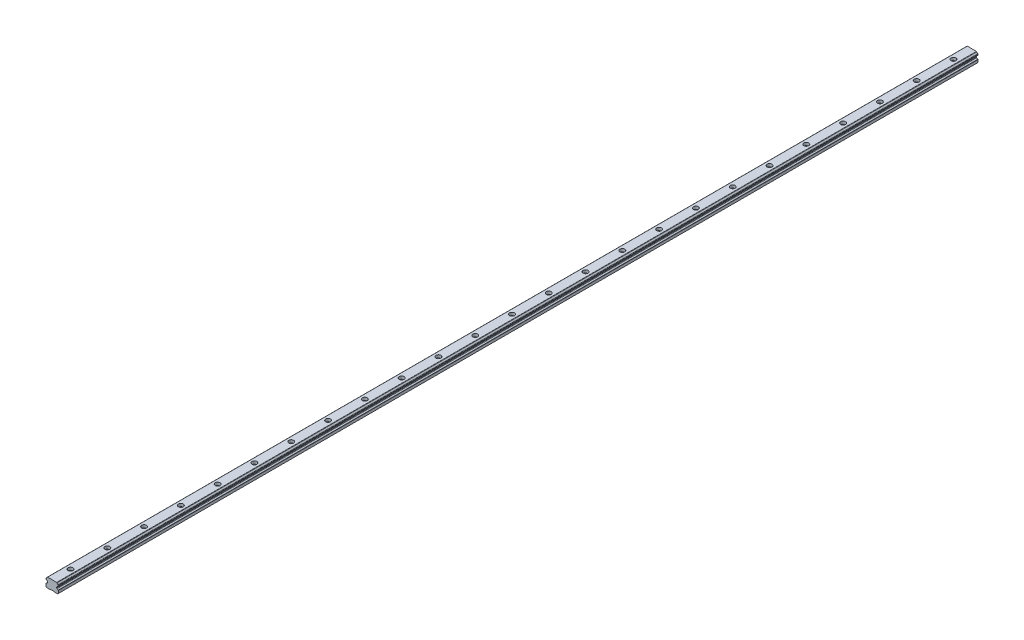
SolidWorks part; units mm, degrees
ref_plane "前视基准面" through (0, 0, 0) normal (0, 0, 1) x (1, 0, 0)
ref_plane "上视基准面" through (0, 0, 0) normal (0, 1, 0) x (1, 0, 0)
ref_plane "右视基准面" through (0, 0, 0) normal (1, 0, 0) x (0, 0, -1)
sketch "草图1" plane through (0, 0, 0) normal (0, 0, 1) x (1, 0, 0)
  line B0 (-9, -15.5) -> (-3, -15.5)
  line B1 (-3, -15.5) -> (-3, -15)
  line B2 (-3, -15) -> (3, -15)
  line B3 (3, -15) -> (3, -15.5)
  line B4 (3, -15.5) -> (9, -15.5)
  line B5 (9, -15.5) -> (10, -14.5)
  line B6 (10, -14.5) -> (10, -10.2831)
  line B7 (9.7572, -9.8543) -> (7.9855, -8.7913)
  line B8 (7.5, -7.9338) -> (7.5, -6.7283)
  line B9 (7.6725, -6.3505) -> (7.7226, -6.3071)
  line B10 (10, -3.8806) -> (10, -2.6194)
  line B11 (7.3806, 0) -> (-7.3806, 0)
  line B12 (-10, -2.6194) -> (-10, -3.8806)
  line B13 (-7.7226, -6.3071) -> (-7.6725, -6.3505)
  line B14 (-7.5, -6.7283) -> (-7.5, -7.9338)
  line B15 (-7.9855, -8.7913) -> (-9.7572, -9.8543)
  line B16 (-10, -10.2831) -> (-10, -14.5)
  line B17 (-10, -14.5) -> (-9, -15.5)
  arc B18 (10, -10.2831) -> (9.7572, -9.8543) centre (9.5, -10.2831) ccw
  arc B19 (7.5, -7.9338) -> (7.9855, -8.7913) centre (8.5, -7.9338) ccw
  arc B20 (7.6725, -6.3505) -> (7.5, -6.7283) centre (8, -6.7283) ccw
  arc B21 (7.7226, -6.3071) -> (7.8835, -6.0363) centre (7.3951, -5.9292) ccw
  arc B22 (9.5938, -4.3718) -> (7.8835, -6.0363) centre (10, -6.5) ccw
  arc B23 (9.5938, -4.3718) -> (10, -3.8806) centre (9.5, -3.8806) ccw
  arc B24 (10, -2.6194) -> (9.5938, -2.1282) centre (9.5, -2.6194) ccw
  arc B25 (7.8718, -0.4063) -> (9.5938, -2.1282) centre (10, 0) ccw
  arc B26 (7.8718, -0.4063) -> (7.3806, 0) centre (7.3806, -0.5) ccw
  arc B27 (-7.3806, 0) -> (-7.8718, -0.4063) centre (-7.3806, -0.5) ccw
  arc B28 (-9.5938, -2.1282) -> (-7.8718, -0.4063) centre (-10, 0) ccw
  arc B29 (-9.5938, -2.1282) -> (-10, -2.6194) centre (-9.5, -2.6194) ccw
  arc B30 (-10, -3.8806) -> (-9.5938, -4.3718) centre (-9.5, -3.8806) ccw
  arc B31 (-7.8835, -6.0363) -> (-9.5938, -4.3718) centre (-10, -6.5) ccw
  arc B32 (-7.8835, -6.0363) -> (-7.7226, -6.3071) centre (-7.3951, -5.9292) ccw
  arc B33 (-7.5, -6.7283) -> (-7.6725, -6.3505) centre (-8, -6.7283) ccw
  arc B34 (-7.9855, -8.7913) -> (-7.5, -7.9338) centre (-8.5, -7.9338) ccw
  arc B35 (-9.7572, -9.8543) -> (-10, -10.2831) centre (-9.5, -10.2831) ccw
sketch_block_instance "块1-1"
sketch_block "块1"
extrude "凸台-拉伸1" add sketch "草图1" along normal mid plane 1500
hole_wizard "打孔尺寸(%根据)内六角圆柱头螺钉的类型1" positions "3D草图1" profile "草图2" counterbore size "M4" standard "GB" end condition up to next
sketch3d "3D草图1"
  line L0 (0, 0, 750) -> (0, 0, -750) construction
  line L1 (7.3806, 0, 750) -> (-7.3806, 0, 750) construction
  line L2 (7.3806, 0, -750) -> (-7.3806, 0, -750) construction
  point P0 (0, 0, 720)
  dimension "D1" = 30
sketch "草图2" plane through (0, 0, 720) normal (1, 0, 0) x (0, 0, 1)
  line L0 (0, 0) -> (0, 15.001)
  line L1 (0, 15.001) -> (2.25, 15.001)
  line L3 (2.25, 15.001) -> (2.25, 4.6)
  line L4 (2.25, 4.6) -> (4, 4.6)
  line L5 (4, 4.6) -> (4, 0)
  line L7 (4, 0) -> (0, 0)
  line L11 (0, -6.35) -> (0, 107.95) construction
  dimension "通孔孔直径" = 4.5
  dimension "通孔孔深度" = 15.001
  dimension "柱形沉头孔直径" = 8
  dimension "柱形沉头孔深度" = 4.6
pattern_linear "阵列(线性)1" count 25 spacing 60 along (0, 0, -1) of "打孔尺寸(%根据)内六角圆柱头螺钉的类型1"
